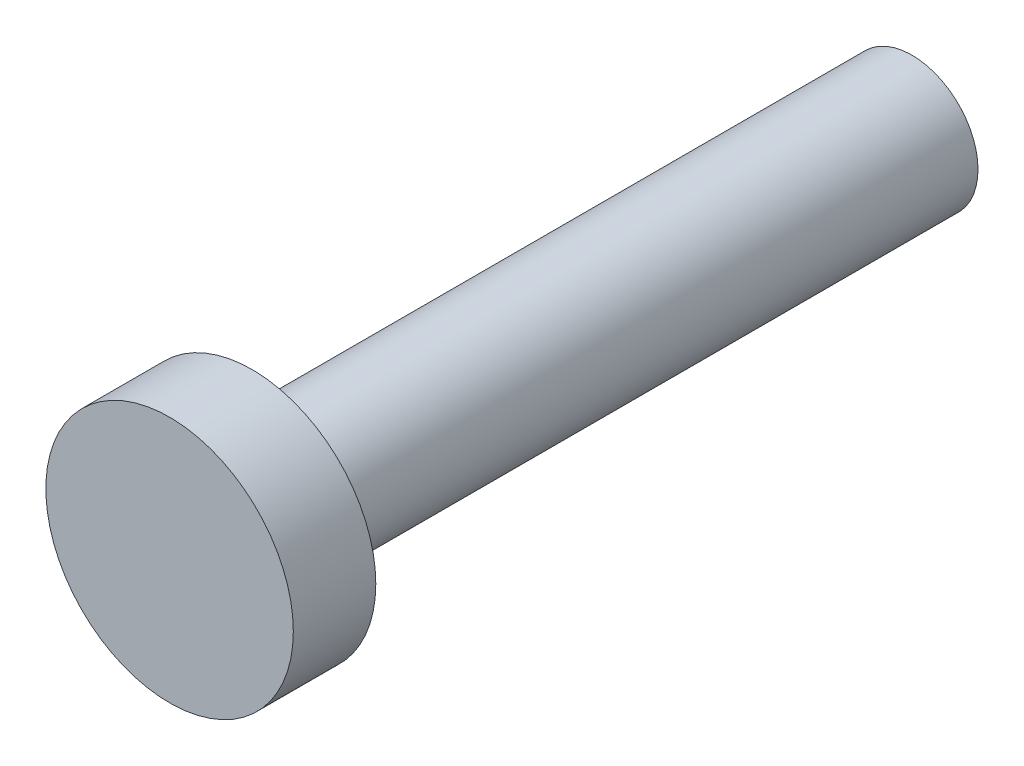
SolidWorks part; units mm, degrees
material "45"
ref_plane "Front" through (0, 0, 0) normal (0, 0, 1) x (1, 0, 0)
ref_plane "Top" through (0, 0, 0) normal (0, 1, 0) x (1, 0, 0)
ref_plane "Right" through (0, 0, 0) normal (1, 0, 0) x (0, 0, -1)
sketch "Sketch1" plane through (0, 0, 0) normal (0, 0, 1) x (1, 0, 0)
  circle A0 centre (0, 0) radius 4
  dimension "D1" = 8
extrude "Boss-Extrude1" add sketch "Sketch1" along normal blind 40
sketch "Sketch2" plane through (0, 0, 40) normal (0, 0, 1) x (1, 0, 0)
  circle A0 centre (0, 0) radius 7.5
  dimension "D1" = 15
extrude "Boss-Extrude2" add sketch "Sketch2" along normal blind 5
equation "\"零件重量\"= IIF ( \"SW-质量\" > 100 , int ( \"SW-质量\" ) , \"SW-质量\" )"
